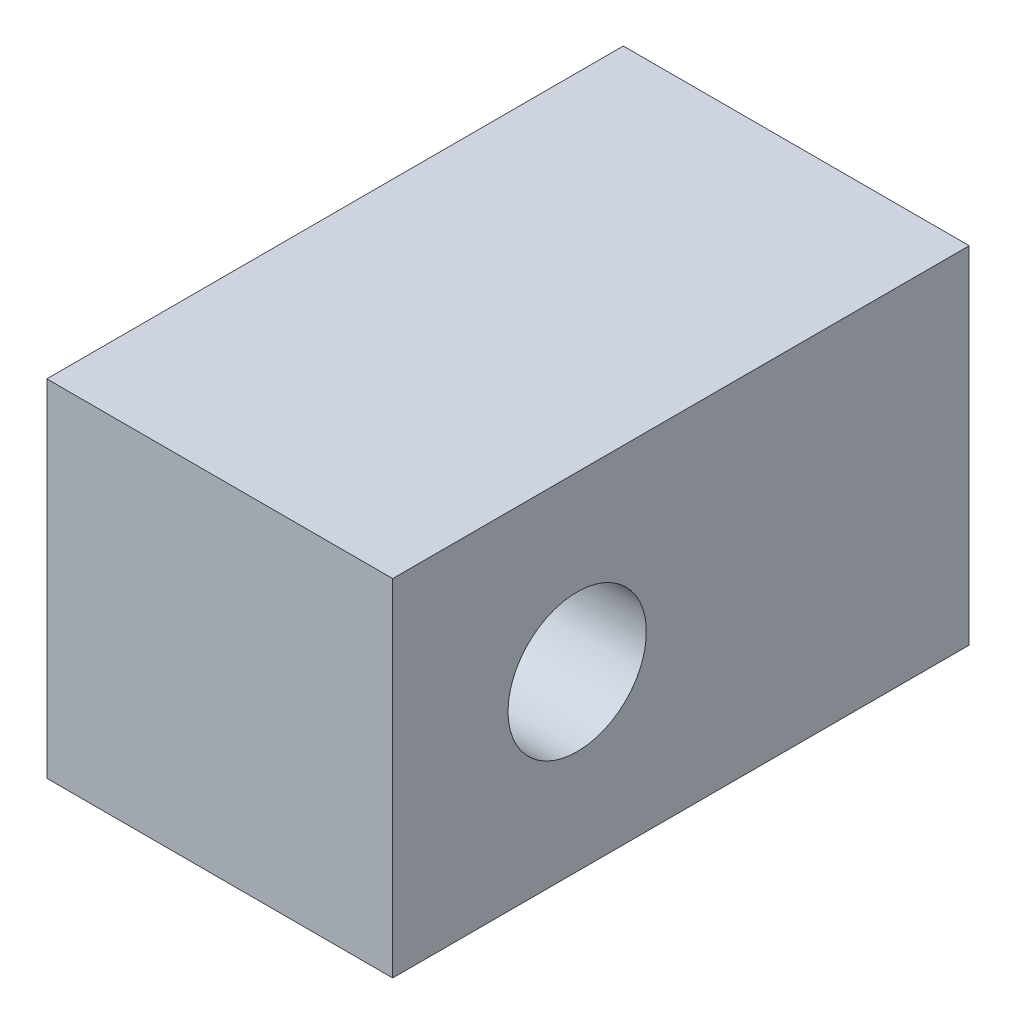
from build123d import *

# Parameters (mm, degrees)
SKETCH1_W               = 15
SKETCH1_H               = 15
BOSS_EXTRUDE1_DEPTH     = 25
CUT_EXTRUDE1_DEPTH      = 31.103986447
CUT_EXTRUDE1_DEPTH_BACK = 31.103986447
SKETCH2_R               = 3


with BuildPart() as part:
    # Sketch1 → Boss-Extrude1 (new body)
    with BuildSketch(Plane.XY):
        Rectangle(SKETCH1_W, SKETCH1_H)
    extrude(amount=BOSS_EXTRUDE1_DEPTH)

    # Sketch2 → Cut-Extrude1 (cut, two sides: drawn at the far end of the back side and taken through both)
    with BuildSketch(Plane.ZY.offset(7.5).offset(-CUT_EXTRUDE1_DEPTH_BACK)):
        with Locations((17, 0)):
            Circle(SKETCH2_R)
    extrude(amount=CUT_EXTRUDE1_DEPTH + CUT_EXTRUDE1_DEPTH_BACK, mode=Mode.SUBTRACT)


solid = part.part
